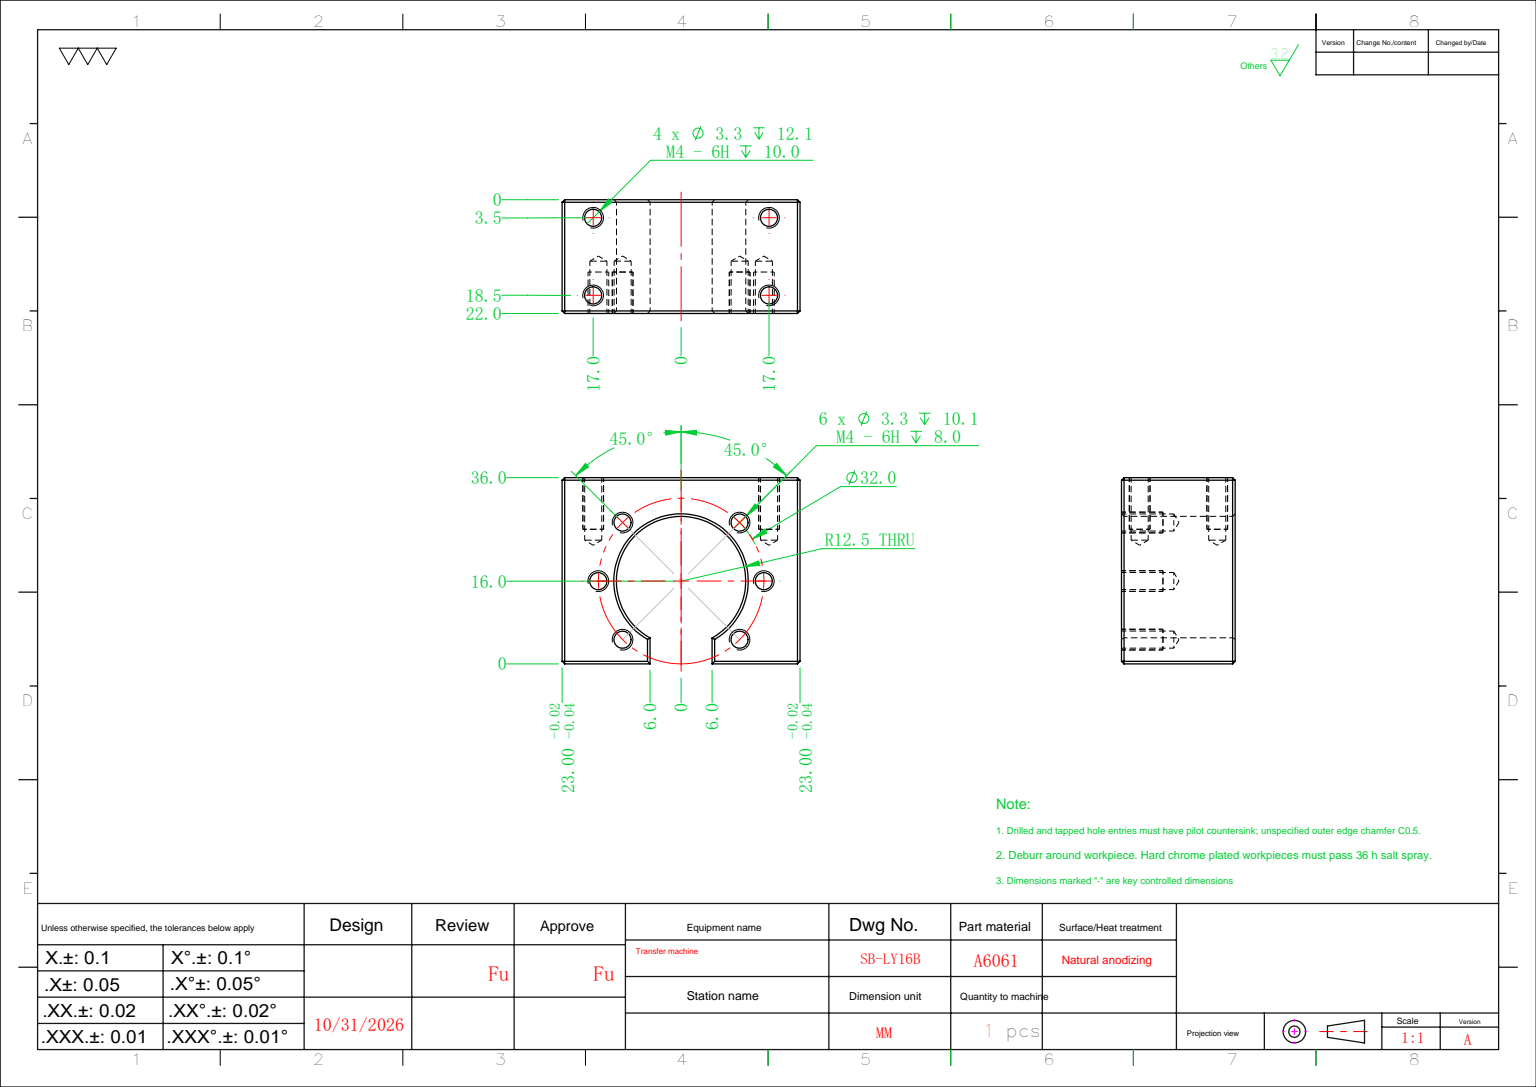
SolidWorks part; units mm, degrees
ref_plane "前视基准面" through (0, 0, 0) normal (0, 0, 1) x (1, 0, 0)
ref_plane "上视基准面" through (0, 0, 0) normal (0, 1, 0) x (1, 0, 0)
ref_plane "右视基准面" through (0, 0, 0) normal (1, 0, 0) x (0, 0, -1)
sketch "草图1" plane through (0, 0, 0) normal (0, 0, 1) x (1, 0, 0)
  line L1 (-23, -18) -> (23, -18)
  line L2 (-23, -18) -> (-23, 18)
  line L3 (-23, 18) -> (23, 18)
  line L4 (23, -18) -> (23, 18)
  line L5 (-23, -18) -> (23, 18) construction
  line L6 (-23, 18) -> (23, -18) construction
  point P0 (0, 0)
  dimension "D1" = 46
  dimension "D2" = 36
extrude "凸台-拉伸1" add sketch "草图1" along normal blind 22
sketch "草图5" plane through (0, 0, 22) normal (0, 0, 1) x (1, 0, 0)
  line L0 (0, 18) -> (0, -21) construction
  line L1 (23, 18) -> (-23, 18) construction
  line L3 (-23, -18) -> (23, -18) construction
  line L5 (-6, -12.9659) -> (-6, -18)
  line L6 (-6, -18) -> (6, -18)
  line L7 (6, -12.9659) -> (6, -18)
  arc A0 (6, -12.9659) -> (-6, -12.9659) centre (0, -2) ccw
  dimension "D1" = 25
  dimension "D2" = 20
  dimension "D3" = 12
extrude "切除-拉伸2" cut sketch "草图5" against normal through all
chamfer "倒角1" distance 0.5 angle 45 20 edges at (-23, 18, 11) (-23, -18, 11) (-23, 0, 22) (0, 18, 22) (-14.5, -18, 22) (14.5, -18, 22) (23, -18, 11) (23, 0, 22) (23, 18, 11) (14.5, -18, 0) (23, 0, 0) (0, 18, 0) (-23, 0, 0) (-14.5, -18, 0) (0, 10.5, 22) (0, 10.5, 0) (-6, -15.4829, 22) (6, -15.4829, 22) (-6, -15.4829, 0) (6, -15.4829, 0)
hole_wizard "M4 螺纹孔1" positions "草图19" profile "草图20" tap size "M4" standard "ISO"
sketch "草图19" plane through (0, 18, 0) normal (0, 1, 0) x (1, 0, 0)
  line L0 (0, -11) -> (0, -26.1171) construction
  line L3 (0, -11) -> (25.2307, -11) construction
  line L4 (0, 0) -> (0, -22) construction
  line L6 (22.5, -22) -> (-22.5, -22) construction
  point P0 (17, -18.5)
  point P4 (17, -3.5)
  point P22 (-17, -3.5)
  point P23 (-17, -18.5)
  dimension "D1" = 15
  dimension "D2" = 34
cosmetic thread "孔螺蚊线8" parameters "D1"=10, "D2"=4
cosmetic thread "孔螺蚊线9" parameters "D1"=10, "D2"=4
cosmetic thread "孔螺蚊线10" parameters "D1"=10, "D2"=4
cosmetic thread "孔螺蚊线11" parameters "D1"=10, "D2"=4
sketch "草图20" plane through (17, 18, 18.5) normal (1, 0, 0) x (0, 0, 1)
  line L0 (0, 0) -> (0, 13.0914)
  line L1 (0, 13.0914) -> (1.65, 12.1)
  line L2 (1.65, 12.1) -> (1.65, 0)
  line L5 (1.65, 0) -> (0, 0)
  line L10 (0, 13.0914) -> (-1.65, 12.1) construction
  line L11 (0, -6.35) -> (0, 107.95) construction
  dimension "螺纹孔钻头直径" = 3.3
  dimension "螺纹孔钻头深度" = 12.1
  dimension "导头角度" = 118
hole_wizard "M4 螺纹孔2" positions "草图21" profile "草图22" tap size "M4" standard "ISO"
sketch "草图21" plane through (0, 0, 0) normal (0, 0, -1) x (-1, 0, 0)
  line L0 (0, -2) -> (-16, -2) construction
  line L2 (0, -2) -> (-11.3137, 9.3137) construction
  line L4 (0, -2) -> (0, 12.8237) construction
  point P0 (-16, -2)
  point P2 (-11.3137, 9.3137)
  point P23 (11.3137, 9.3137)
  point P24 (16, -2)
  point P25 (-11.3137, -13.3137)
  point P28 (11.3137, -13.3137)
  dimension "D1" = 32
  dimension "D2" = 45
sketch "草图22" plane through (16, -2, 0) normal (1, 0, 0) x (0, 1, 0)
  line L0 (0, 0) -> (0, 11.0914)
  line L1 (0, 11.0914) -> (1.65, 10.1)
  line L2 (1.65, 10.1) -> (1.65, 0)
  line L5 (1.65, 0) -> (0, 0)
  line L10 (0, 11.0914) -> (-1.65, 10.1) construction
  line L11 (0, -6.35) -> (0, 107.95) construction
  dimension "螺纹孔钻头直径" = 3.3
  dimension "螺纹孔钻头深度" = 10.1
  dimension "导头角度" = 118
cosmetic thread "孔螺蚊线12" parameters "D1"=8, "D2"=4
cosmetic thread "孔螺蚊线13" parameters "D1"=8, "D2"=4
cosmetic thread "孔螺蚊线14" parameters "D1"=8, "D2"=4
cosmetic thread "孔螺蚊线15" parameters "D1"=8, "D2"=4
cosmetic thread "孔螺蚊线16" parameters "D1"=8, "D2"=4
cosmetic thread "孔螺蚊线17" parameters "D1"=8, "D2"=4
